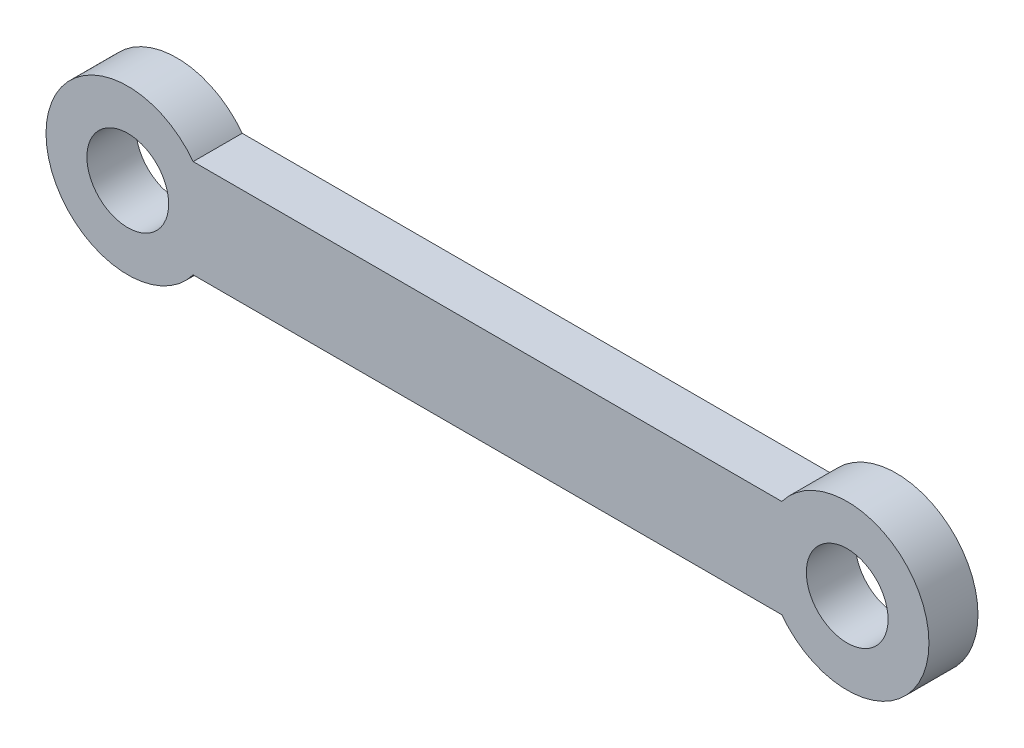
from build123d import *

# Parameters (mm, degrees)
SKETCH1_R           = 2.5
BOSS_EXTRUDE1_DEPTH = 3


with BuildPart() as part:
    # Sketch1 → Boss-Extrude1 (new body)
    with BuildSketch(Plane.XY):
        with BuildLine():
            Line((4, 3), (40, 3))
            ThreePointArc((40, 3), (49, 0), (40, -3))
            Line((40, -3), (4, -3))
            ThreePointArc((4, -3), (-5, 0), (4, 3))
        make_face()
        Circle(SKETCH1_R, mode=Mode.SUBTRACT)
        with Locations((44, 0)):
            Circle(SKETCH1_R, mode=Mode.SUBTRACT)
    extrude(amount=BOSS_EXTRUDE1_DEPTH)


solid = part.part
